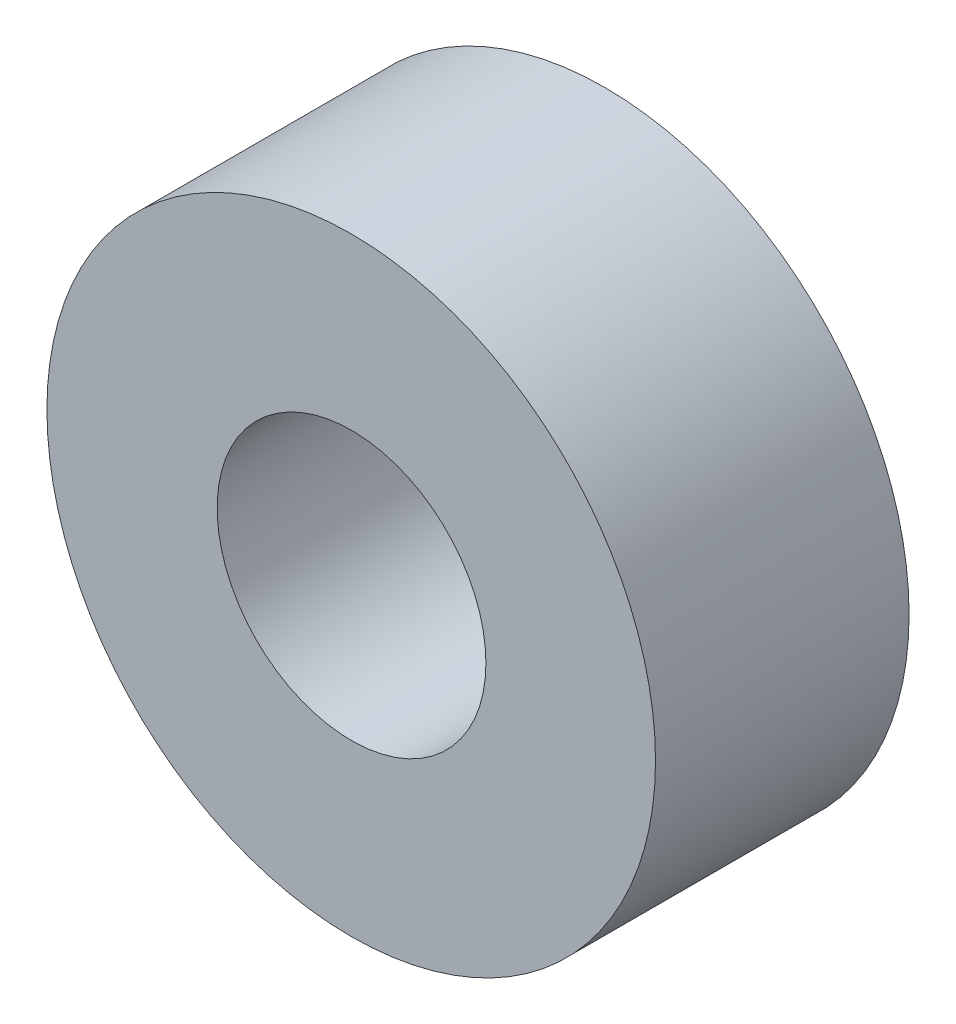
from build123d import *

# Parameters (mm, degrees)
SKETCH1_R              = 30
BOSS_EXTRUDE1_DEPTH    = 25
M30_TAPPED_HOLE3_D     = 26.5
M30_TAPPED_HOLE3_DEPTH = 70.5
M30_TAPPED_HOLE3_TIP   = 7.961403202


with BuildPart() as part:
    # Sketch1 → Boss-Extrude1 (new body)
    with BuildSketch(Plane.XY):
        Circle(SKETCH1_R)
    extrude(amount=BOSS_EXTRUDE1_DEPTH)

    # M30 Tapped Hole3
    with Locations(Plane(origin=(0.031473792, -0.003286401, 25), x_dir=(1, 0, 0), z_dir=(0, 0, 1))):
        with Locations((0, 0)):
            Hole(M30_TAPPED_HOLE3_D / 2, depth=M30_TAPPED_HOLE3_DEPTH)
            with Locations((0, 0, -(M30_TAPPED_HOLE3_DEPTH + M30_TAPPED_HOLE3_TIP / 2))):  # 118° drill point
                Cone(0, M30_TAPPED_HOLE3_D / 2, M30_TAPPED_HOLE3_TIP, mode=Mode.SUBTRACT)


solid = part.part
